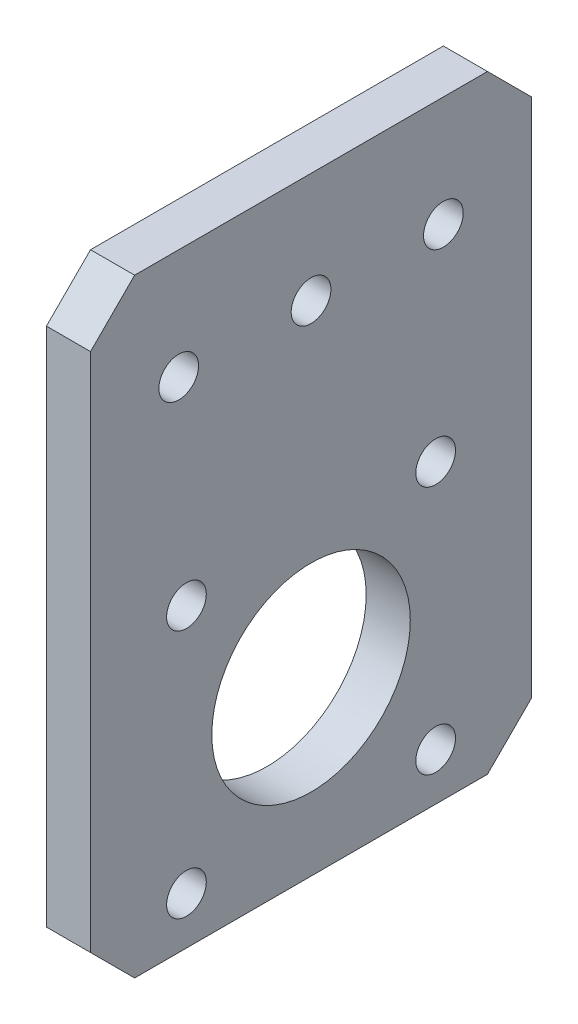
from build123d import *

# Parameters (mm, degrees)
SKETCH_1_W               = 100
SKETCH_1_H               = 138
EXTRUDE_1_DEPTH          = 10
HOLE_WIZARD_9_0_9_1_D    = 9
SKETCH_4_R               = 22.5
CUT_EXTRUDE_1_DEPTH      = 10
HOLE_WIZARD_9_0_9_2_D    = 9
PATTERN_CIRCULAR_1_COUNT = 4
CHAMFER_1_SIZE           = 10


with BuildPart() as part:
    # 草图1 → 凸台-拉伸1 (new body)
    with BuildSketch(Plane(origin=(0, 0, 0), x_dir=(0, 0, -1), z_dir=(1, 0, 0))):
        Rectangle(SKETCH_1_W, SKETCH_1_H)
    extrude(amount=EXTRUDE_1_DEPTH)

    # Ø9.0 (9) 直径孔1 (through all)
    with Locations(Plane(origin=(10, 0, 0), x_dir=(0, 0, -1), z_dir=(1, 0, 0))):
        with Locations((-30, 44), (0, 44), (30, 44)):
            Hole(HOLE_WIZARD_9_0_9_1_D / 2)

    # 草图4 → 切除-拉伸1 (cut)
    with BuildSketch(Plane(origin=(10, 0, 0), x_dir=(0, 0, -1), z_dir=(1, 0, 0))):
        with Locations((0, -30)):
            Circle(SKETCH_4_R)
    extrude(amount=-CUT_EXTRUDE_1_DEPTH, mode=Mode.SUBTRACT)

    # Ø9.0 (9) 直径孔2 (through all)
    with Locations(Plane(origin=(10, 0, 0), x_dir=(0, 0, -1), z_dir=(1, 0, 0))):
        with Locations((-28.25, -1.75)):
            hole_wizard_9_0_9_2 = Hole(HOLE_WIZARD_9_0_9_2_D / 2)

    # 阵列(圆周)1: Ø9.0 (9) 直径孔2 ×4 about axis
    pattern_circular_1_axis = Axis((0, -30, 0), (1, 0, 0))
    for i in range(1, PATTERN_CIRCULAR_1_COUNT):
        add(hole_wizard_9_0_9_2.rotate(pattern_circular_1_axis, i * 360 / PATTERN_CIRCULAR_1_COUNT), mode=Mode.SUBTRACT)

    # 倒角1
    chamfer_1_edges = [part.edges().sort_by_distance(p)[0] for p in [
        (5, -69, -50),
        (5, -69, 50),
        (5, 69, 50),
        (5, 69, -50),
    ]]
    chamfer(chamfer_1_edges, length=CHAMFER_1_SIZE)


solid = part.part
